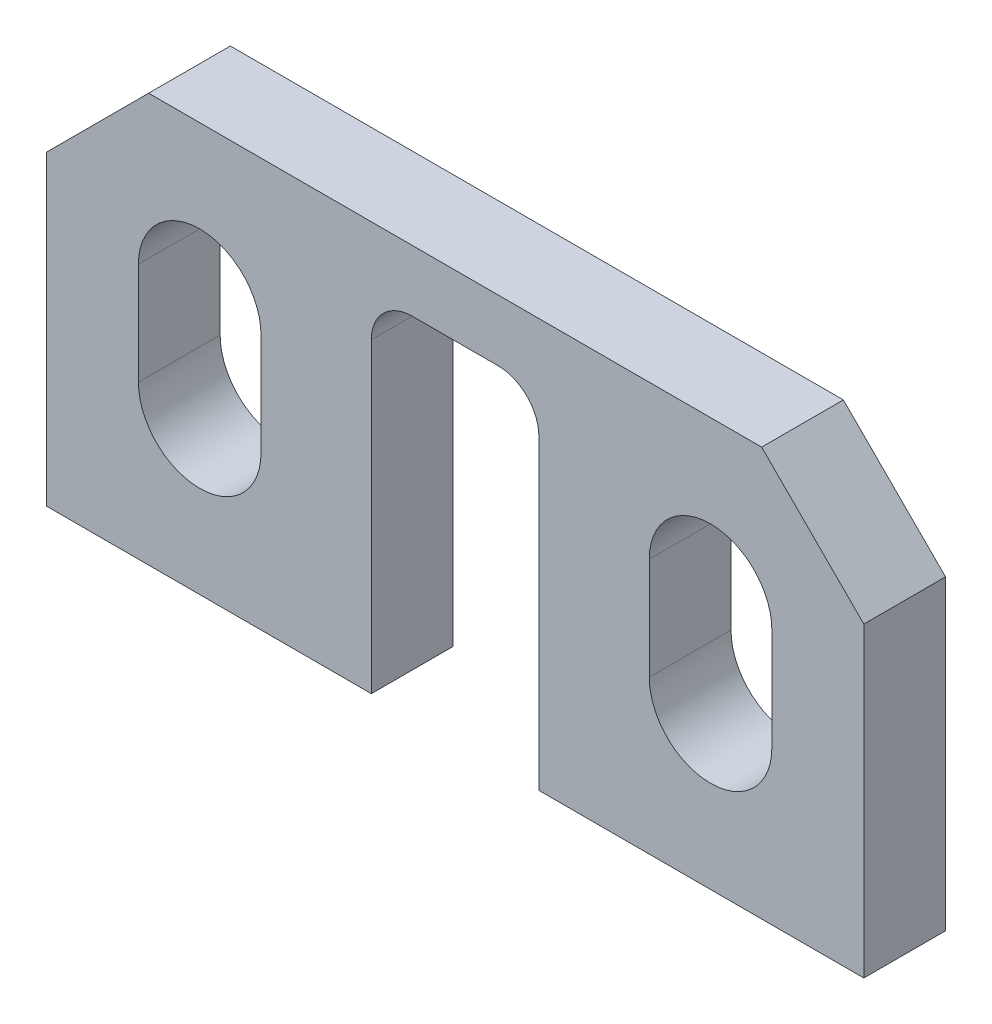
from build123d import *

# Parameters (mm, degrees)
SKETCH_1_W             = 40
SKETCH_1_H             = 20
EXTRUDE_1_DEPTH        = 4
CUT_EXTRUDE_1_DEPTH    = 23.715633383
CHAMFER_1_SIZE         = 5
SKETCH_3_R             = 3
CUT_EXTRUDE_2_DEPTH    = 23.715633383
CUT_EXTRUDE_3_DEPTH    = 23.715633383
PATTERN_LINEAR_1_COUNT = 2
PATTERN_LINEAR_1_PITCH = 25
FILLET_1_R             = 2


with BuildPart() as part:
    # 草图1 → 凸台-拉伸1 (new body)
    with BuildSketch(Plane.XY):
        Rectangle(SKETCH_1_W, SKETCH_1_H)
    extrude(amount=EXTRUDE_1_DEPTH)

    # 草图2 → 切除-拉伸1 (cut, through all)
    with BuildSketch(Plane.XY.offset(4)):
        with BuildLine():
            Line((4.1, 7), (4.1, -18.947287746))
            ThreePointArc((4.1, -18.947287746), (0, -23.047287746), (-4.1, -18.947287746))
            Line((-4.1, -18.947287746), (-4.1, 7))
            Line((-4.1, 7), (4.1, 7))
        make_face()
    extrude(amount=-CUT_EXTRUDE_1_DEPTH, mode=Mode.SUBTRACT)

    # 倒角1
    chamfer_1_edges = [part.edges().sort_by_distance(p)[0] for p in [
        (-20, 10, 2),
        (20, 10, 2),
    ]]
    chamfer(chamfer_1_edges, length=CHAMFER_1_SIZE)

    # 草图3 → 切除-拉伸2 (cut, through all)
    with BuildSketch(Plane.XY.offset(4)):
        with Locations((-12.5, 0)):
            Circle(SKETCH_3_R)
        with Locations((12.5, 0)):
            Circle(SKETCH_3_R)
    extrude(amount=-CUT_EXTRUDE_2_DEPTH, mode=Mode.SUBTRACT)

    # 草图5 → 切除-拉伸3 (cut, through all)
    with BuildSketch(Plane.XY.offset(4)):
        with BuildLine():
            Line((-9.5, 2.5), (-9.5, -2.5))
            ThreePointArc((-9.5, -2.5), (-12.5, -5.5), (-15.5, -2.5))
            Line((-15.5, -2.5), (-15.5, 2.5))
            ThreePointArc((-15.5, 2.5), (-12.5, 5.5), (-9.5, 2.5))
        make_face()
    cut_extrude_3 = extrude(amount=-CUT_EXTRUDE_3_DEPTH, mode=Mode.SUBTRACT)

    # 阵列(线性)1: 切除-拉伸3 ×2
    with Locations(*[(i * PATTERN_LINEAR_1_PITCH, 0, 0) for i in range(1, PATTERN_LINEAR_1_COUNT)]):
        add(cut_extrude_3, mode=Mode.SUBTRACT)

    # 圆角1
    fillet_1_edges = [part.edges().sort_by_distance(p)[0] for p in [
        (4.1, 7, 2),
        (-4.1, 7, 2),
    ]]
    fillet(fillet_1_edges, radius=FILLET_1_R)


solid = part.part
